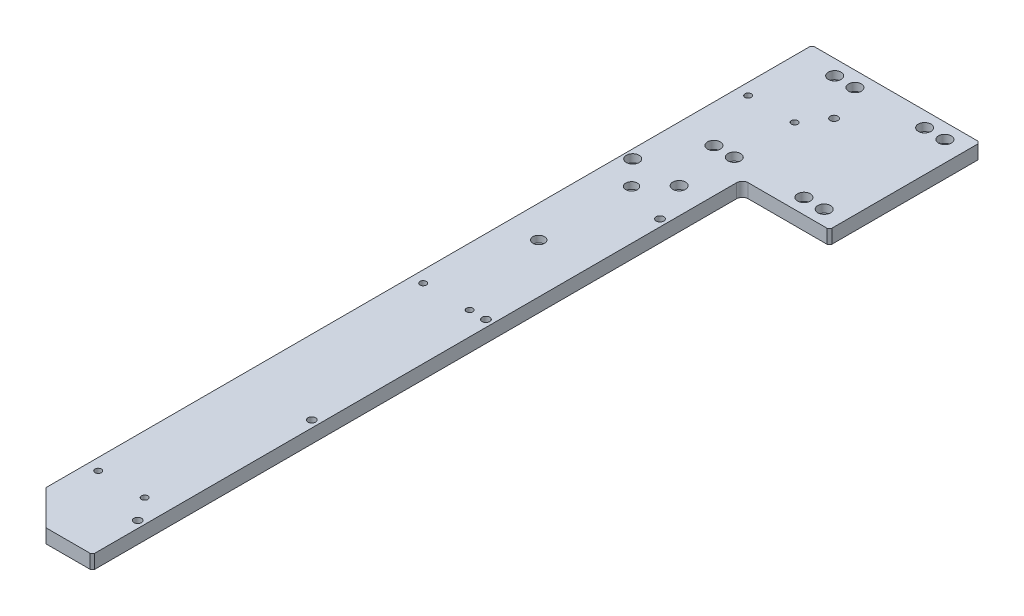
SolidWorks part; units mm, degrees
material "A6061"
ref_plane "前基準面" through (0, 0, 0) normal (0, 0, 1) x (1, 0, 0)
ref_plane "上基準面" through (0, 0, 0) normal (0, 1, 0) x (1, 0, 0)
ref_plane "右基準面" through (0, 0, 0) normal (1, 0, 0) x (0, 0, -1)
sketch "草图1" plane through (0, 0, 0) normal (0, 1, 0) x (1, 0, 0)
  line L1 (-72.5, 345) -> (72.5, 345)
  line L2 (-72.5, 345) -> (-72.5, -345)
  line L3 (-72.5, -345) -> (72.5, -345)
  line L4 (72.5, 345) -> (72.5, -345)
  line L5 (-72.5, 345) -> (72.5, -345) construction
  line L6 (-72.5, -345) -> (72.5, 345) construction
  point P0 (0, 0)
  dimension "D1" = 690
  dimension "D2" = 145
extrude "凸台-拉伸1" add sketch "草图1" along normal mid plane 12
sketch "草图2" plane through (0, 6, 0) normal (0, 1, 0) x (1, 0, 0)
  line L0 (72.5, -345) -> (72.5, 345) construction
  line L1 (72.5, -345) -> (-2.5, -345)
  line L2 (72.5, -345) -> (72.5, 215)
  line L3 (72.5, 215) -> (2.5, 215)
  line L4 (-2.5, -345) -> (-2.5, 210)
  line L5 (72.5, 345) -> (-72.5, 345) construction
  arc A0 (2.5, 215) -> (-2.5, 210) centre (2.5, 210) ccw
  dimension "D4" = 5
  dimension "D1" = 75
  dimension "D3" = 130
extrude "切除-拉伸1" cut sketch "草图2" against normal through all
chamfer "倒角1" distance 2 angle 45 4 edges at (-72.5, 0, -345) (72.5, 0, -345) (72.5, 0, -215) (-2.5, 0, 345)
hole_wizard "打孔尺寸(%根据)内六角圆柱头螺钉的类型1" positions "草图3" profile "草图4" counterbore size "M6" standard "GB" end condition through all
sketch "草图3" plane through (0, 6, 0) normal (0, 1, 0) x (1, 0, 0)
  line L0 (72.5, 280) -> (7.5, 280) construction
  line L1 (72.5, 217) -> (72.5, 343) construction
  line L2 (7.5, 280) -> (7.5, 345) construction
  point P0 (-40, 228)
  point P2 (-22.5, 228)
  point P14 (37.5, 228)
  point P15 (55, 228)
  point P16 (55, 332)
  point P17 (37.5, 332)
  point P18 (-22.5, 332)
  point P19 (-40, 332)
  dimension "D1" = 104
  dimension "D2" = 17.5
  dimension "D3" = 95
  dimension "D4" = 65
sketch "草图4" plane through (-40, 6, -228) normal (1, 0, 0) x (0, 0, 1)
  line L0 (0, 0) -> (0, 12)
  line L1 (0, 12) -> (3.3, 12)
  line L3 (3.3, 12) -> (3.3, 6.8)
  line L4 (3.3, 6.8) -> (5.5, 6.8)
  line L5 (5.5, 6.8) -> (5.5, 0)
  line L7 (5.5, 0) -> (0, 0)
  line L11 (0, -6.35) -> (0, 107.95) construction
  dimension "通孔孔直径" = 6.6
  dimension "通孔孔深度" = 12
  dimension "柱形沉头孔直径" = 11
  dimension "柱形沉头孔深度" = 6.8
hole_wizard "打孔尺寸(%根据)内六角圆柱头螺钉的类型2" positions "草图5" profile "草图6" counterbore size "M6" standard "GB" end condition through all
sketch "草图5" plane through (0, -6, 0) normal (0, -1, 0) x (-1, 0, 0)
  line L0 (2.5, 210) -> (2.5, -343) construction
  point P0 (8.5, 300)
  point P7 (8.5, 150)
  point P8 (8.5, 0)
  point P9 (8.5, -150)
  point P10 (8.5, -300)
  dimension "D2" = 150
  dimension "D3" = 6
  dimension "D1" = 5
sketch "草图6" plane through (-8.5, -6, -300) normal (1, 0, 0) x (0, 0, -1)
  line L0 (0, 0) -> (0, 12)
  line L1 (0, 12) -> (3.3, 12)
  line L3 (3.3, 12) -> (3.3, 6.8)
  line L4 (3.3, 6.8) -> (5.5, 6.8)
  line L5 (5.5, 6.8) -> (5.5, 0)
  line L7 (5.5, 0) -> (0, 0)
  line L11 (0, -6.35) -> (0, 107.95) construction
  dimension "通孔孔直径" = 6.6
  dimension "通孔孔深度" = 12
  dimension "柱形沉头孔直径" = 11
  dimension "柱形沉头孔深度" = 6.8
hole_wizard "打孔尺寸(%根据)内六角圆柱头螺钉的类型3" positions "草图7" profile "草图8" counterbore size "M5" standard "GB" end condition through all
sketch "草图7" plane through (0, -6, 0) normal (0, -1, 0) x (-1, 0, 0)
  line L0 (72.5, 343) -> (72.5, -345) construction
  line L1 (22.5, 280) -> (-72.5, 280) construction
  line L2 (-72.5, 217) -> (-72.5, 343) construction
  point P0 (22.5, 280)
  point P2 (62.5, 280)
  point P8 (22.5, 0)
  point P9 (62.5, 0)
  point P10 (22.5, -280)
  point P11 (62.5, -280)
  dimension "D2" = 40
  dimension "D3" = 280
  dimension "D4" = 10
  dimension "D1" = 3
sketch "草图8" plane through (-22.5, -6, -280) normal (1, 0, 0) x (0, 0, -1)
  line L0 (0, 0) -> (0, 12)
  line L1 (0, 12) -> (2.75, 12)
  line L3 (2.75, 12) -> (2.75, 5.7)
  line L4 (2.75, 5.7) -> (5, 5.7)
  line L5 (5, 5.7) -> (5, 0)
  line L7 (5, 0) -> (0, 0)
  line L11 (0, -6.35) -> (0, 107.95) construction
  dimension "通孔孔直径" = 5.5
  dimension "通孔孔深度" = 12
  dimension "柱形沉头孔直径" = 10
  dimension "柱形沉头孔深度" = 5.7
hole_wizard "M5 螺纹孔1" positions "草图9" profile "草图10" tap size "M5" standard "GB"
sketch "草图9" plane through (0, 0, -345) normal (0, 0, -1) x (-1, 0, 0)
  line L1 (-72.5, -6) -> (-72.5, 6) construction
  point P0 (-7.5, 0)
  point P2 (-47.5, 0)
  dimension "D1" = 40
  dimension "D2" = 25
sketch "草图10" plane through (7.5, 0, -345) normal (1, 0, 0) x (0, 1, 0)
  line L0 (0, 0) -> (0, 13.6618)
  line L1 (0, 13.6618) -> (2.1, 12.4)
  line L2 (2.1, 12.4) -> (2.1, 0)
  line L5 (2.1, 0) -> (0, 0)
  line L10 (0, 13.6618) -> (-2.1, 12.4) construction
  line L11 (0, -6.35) -> (0, 107.95) construction
  dimension "螺纹孔钻头直径" = 4.2
  dimension "螺纹孔钻头深度" = 12.4
  dimension "导头角度" = 118
cosmetic thread "孔螺蚊线1" parameters "D1"=10, "D2"=5
cosmetic thread "孔螺蚊线2" parameters "D1"=10, "D2"=5
hole_wizard "打孔尺寸(%根据)内六角圆柱头螺钉的类型4" positions "草图11" profile "草图12" counterbore size "M6" standard "GB" end condition through all
sketch "草图11" plane through (0, 6, 0) normal (0, 1, 0) x (1, 0, 0)
  line L0 (-72.5, 343) -> (-72.5, -345) construction
  line L1 (70.5, 345) -> (-70.5, 345) construction
  point P0 (-65, 183)
  point P2 (-25, 183)
  dimension "D1" = 7.5
  dimension "D2" = 40
  dimension "D3" = 162
sketch "草图12" plane through (-65, 6, -183) normal (1, 0, 0) x (0, 0, 1)
  line L0 (0, 0) -> (0, 12)
  line L1 (0, 12) -> (3.3, 12)
  line L3 (3.3, 12) -> (3.3, 6.8)
  line L4 (3.3, 6.8) -> (5.5, 6.8)
  line L5 (5.5, 6.8) -> (5.5, 0)
  line L7 (5.5, 0) -> (0, 0)
  line L11 (0, -6.35) -> (0, 107.95) construction
  dimension "通孔孔直径" = 6.6
  dimension "通孔孔深度" = 12
  dimension "柱形沉头孔直径" = 11
  dimension "柱形沉头孔深度" = 6.8
hole_wizard "打孔尺寸(%根据)内六角圆柱头螺钉的类型5" positions "草图13" profile "草图14" counterbore size "M5" standard "GB" end condition through all
sketch "草图13" plane through (0, 6, 0) normal (0, 1, 0) x (1, 0, 0)
  line L0 (-25, 183) -> (-65, 183) construction
  line L2 (-45, 183) -> (-45, 187.3074) construction
  point P0 (-45, 162)
  point P2 (-45, 82)
  dimension "D1" = 21
  dimension "D2" = 80
sketch "草图14" plane through (-45, 6, -162) normal (1, 0, 0) x (0, 0, 1)
  line L0 (0, 0) -> (0, 12)
  line L1 (0, 12) -> (2.75, 12)
  line L3 (2.75, 12) -> (2.75, 5.7)
  line L4 (2.75, 5.7) -> (5, 5.7)
  line L5 (5, 5.7) -> (5, 0)
  line L7 (5, 0) -> (0, 0)
  line L11 (0, -6.35) -> (0, 107.95) construction
  dimension "通孔孔直径" = 5.5
  dimension "通孔孔深度" = 12
  dimension "柱形沉头孔直径" = 10
  dimension "柱形沉头孔深度" = 5.7
chamfer "倒角2" distance 30 angle 45 1 edges at (-72.5, 0, 345)
